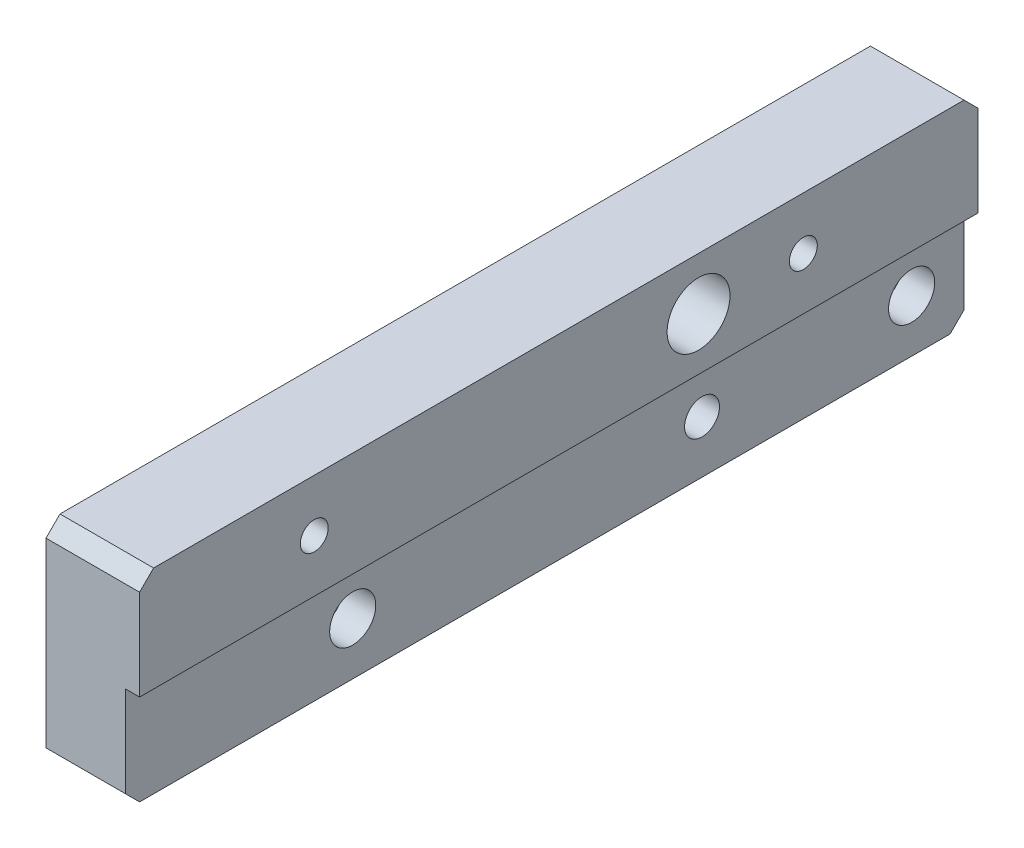
SolidWorks part; units mm, degrees
material "45#"
ref_plane "Front Plane" through (0, 0, 0) normal (0, 0, 1) x (1, 0, 0)
ref_plane "Top Plane" through (0, 0, 0) normal (0, 1, 0) x (1, 0, 0)
ref_plane "Right Plane" through (0, 0, 0) normal (1, 0, 0) x (0, 0, -1)
sketch "Sketch1" plane through (0, 0, 0) normal (1, 0, 0) x (0, 0, -1)
  line L1 (-60, -15) -> (60, -15)
  line L2 (-60, -15) -> (-60, 15)
  line L3 (-60, 15) -> (60, 15)
  line L4 (60, -15) -> (60, 15)
  line L5 (-60, -15) -> (60, 15) construction
  line L6 (-60, 15) -> (60, -15) construction
  point P0 (0, 0)
  dimension "D1" = 120
  dimension "D2" = 30
extrude "Boss-Extrude1" add sketch "Sketch1" along normal blind 13.4
sketch "Sketch2" plane through (13.4, 0, 0) normal (1, 0, 0) x (0, 0, -1)
  line L1 (-60, -15) -> (60, -15)
  line L2 (-60, -15) -> (-60, 0)
  line L3 (-60, 0) -> (60, 0)
  line L4 (60, -15) -> (60, 0)
  line L5 (-60, -15) -> (60, -15) construction
  line L6 (60, -15) -> (60, 15) construction
  line L7 (-60, 15) -> (-60, -15) construction
  dimension "D1" = 15
extrude "Cut-Extrude1" cut sketch "Sketch2" against normal blind 2
hole_wizard "Hole1" positions "Sketch3" profile "Sketch4" legacy
sketch "Sketch3" plane through (0, 0, 0) normal (-1, 0, 0) x (0, 0, 1)
  line L0 (60, 7.5) -> (-60, 7.5) construction
  line L1 (60, 15) -> (60, -15) construction
  line L2 (-60, -15) -> (-60, 15) construction
  line L4 (-60, 15) -> (60, 15) construction
  point P0 (35, 7.5)
  point P2 (-35, 7.5)
  dimension "D1" = 7.5
  dimension "D2" = 70
  dimension "D3" = 25
sketch "Sketch4" plane through (0, 7.5, 35) normal (0, 1, 0) x (0, 0, 1)
  line L0 (0, 0) -> (0, 20)
  line L1 (0, 20) -> (2, 20)
  line L2 (2, 20) -> (2, 8.7017)
  line L3 (2, 8.7017) -> (4, 7.5)
  line L4 (4, 7.5) -> (4, 0)
  line L5 (4, 0) -> (0, 0)
  line L6 (0, -6.13) -> (0, 109.2824) construction
  line L7 (-2, 8.7017) -> (-4, 7.5) construction
  line L8 (0, 20) -> (-2, 20) construction
  dimension "直径" = 4
  dimension "深度" = 20
  dimension "沉头坑直径" = 8
  dimension "沉头坑深度" = 7.5
  dimension "导头角度" = 118
hole_wizard "M8 Clearance Hole1" positions "Sketch7" profile "Sketch8" hole size "M8" standard "GB" end condition through all
sketch "Sketch7" plane through (13.4, 0, 0) normal (1, 0, 0) x (0, 0, -1)
  line L0 (-35, 7.5) -> (35, 7.5) construction
  circle A0 centre (35, 7.5) radius 2 construction
  point P7 (20, 7.5)
  dimension "D1" = 15
sketch "Sketch8" plane through (13.4, 7.5, -20) normal (0, 1, 0) x (0, 0, -1)
  line L0 (0, 0) -> (0, 13.4)
  line L1 (0, 13.4) -> (4.5, 13.4)
  line L2 (4.5, 13.4) -> (4.5, 0)
  line L5 (4.5, 0) -> (0, 0)
  line L11 (0, -6.35) -> (0, 107.95) construction
  dimension "通孔孔直径" = 9
  dimension "通孔孔深度" = 13.4
chamfer "Chamfer1" distance 2 angle 45 4 edges at (5.7, -15, -60) (6.7, 15, -60) (5.7, -15, 60) (6.7, 15, 60)
hole_wizard "CBORE for M5 Hexagon socket head cap screws1" positions "Sketch9" profile "Sketch10" counterbore size "M5" standard "GB"
sketch "Sketch9" plane through (13, 0, 0) normal (1, 0, 0) x (0, 0, -1)
  point P0 (-50, 7.5)
  point P3 (50, 7.5)
sketch "Sketch10" plane through (13, 7.5, 50) normal (0, 1, 0) x (0, 0, -1)
  line L0 (0, 0) -> (0, 13)
  line L1 (0, 13) -> (2.75, 13)
  line L3 (2.75, 13) -> (2.75, 5.7)
  line L4 (2.75, 5.7) -> (5, 5.7)
  line L5 (5, 5.7) -> (5, 0)
  line L7 (5, 0) -> (0, 0)
  line L11 (0, -6.35) -> (0, 107.95) construction
  dimension "通孔孔直径" = 5.5
  dimension "通孔孔深度" = 13
  dimension "柱形沉头孔直径" = 10
  dimension "柱形沉头孔深度" = 5.7
hole_wizard "CBORE for M6 Hexagon socket head cap screws1" positions "Sketch11" profile "Sketch12" counterbore size "M6" standard "GB" end condition through all
sketch "Sketch11" plane through (0, 0, 0) normal (-1, 0, 0) x (0, 0, 1)
  point P0 (-52.5, -7.5)
  point P3 (27.5, -7.5)
sketch "Sketch12" plane through (0, -7.5, -52.5) normal (0, 1, 0) x (0, 0, 1)
  line L0 (0, 0) -> (0, 13.4)
  line L1 (0, 13.4) -> (3.3, 13.4)
  line L3 (3.3, 13.4) -> (3.3, 6.8)
  line L4 (3.3, 6.8) -> (5.5, 6.8)
  line L5 (5.5, 6.8) -> (5.5, 0)
  line L7 (5.5, 0) -> (0, 0)
  line L11 (0, -6.35) -> (0, 107.95) construction
  dimension "通孔孔直径" = 6.6
  dimension "通孔孔深度" = 13.4
  dimension "柱形沉头孔直径" = 11
  dimension "柱形沉头孔深度" = 6.8
hole_wizard "Ø5.0mm blind hole 1" positions "Sketch13" profile "Sketch14" hole size "Ø5.0" standard "GB" end condition through all
sketch "Sketch13" plane through (0, 0, 0) normal (-1, 0, 0) x (0, 0, 1)
  point P0 (-22.5, -7.5)
sketch "Sketch14" plane through (0, -7.5, -22.5) normal (0, 1, 0) x (0, 0, 1)
  line L0 (0, 0) -> (0, 13.4)
  line L1 (0, 13.4) -> (2.5, 13.4)
  line L2 (2.5, 13.4) -> (2.5, 0)
  line L5 (2.5, 0) -> (0, 0)
  line L11 (0, -6.35) -> (0, 107.95) construction
  dimension "通孔孔直径" = 5
  dimension "通孔孔深度" = 13.4
